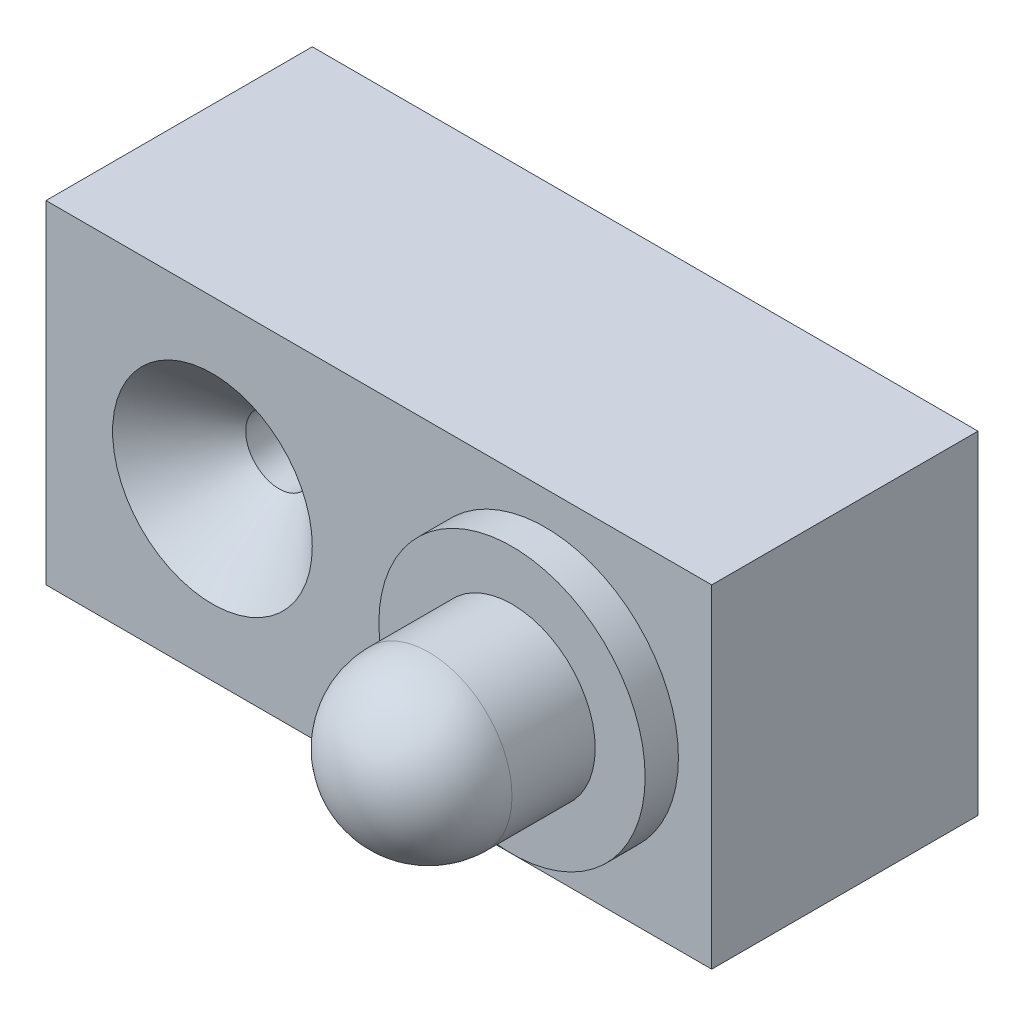
SolidWorks part; units mm, degrees
ref_plane "前视基准面" through (0, 0, 0) normal (0, 0, 1) x (1, 0, 0)
ref_plane "上视基准面" through (0, 0, 0) normal (0, 1, 0) x (1, 0, 0)
ref_plane "右视基准面" through (0, 0, 0) normal (1, 0, 0) x (0, 0, -1)
sketch "草图1" plane through (0, 0, 0) normal (0, 0, 1) x (1, 0, 0)
  line L1 (0, 0) -> (20, 0)
  line L2 (0, 0) -> (0, 10)
  line L3 (0, 10) -> (20, 10)
  line L4 (20, 0) -> (20, 10)
extrude "凸台-拉伸1" add sketch "草图1" along normal blind 8
sketch "草图2" plane through (0, 0, 8) normal (0, 0, 1) x (1, 0, 0)
  line L0 (0, 0) -> (20, 0) construction
  line L1 (0, 10) -> (0, 0) construction
  circle A0 centre (5, 5) radius 1
  dimension "D1" = 2
  dimension "D2" = 5
  dimension "D3" = 5
extrude "切除-拉伸1" cut sketch "草图2" against normal blind 8
chamfer "倒角1" distance 2 angle 45 1 edges at (6, 5, 8)
sketch "草图3" plane through (0, 0, 8) normal (0, 0, 1) x (1, 0, 0)
  line L0 (20, 0) -> (20, 10) construction
  circle A0 centre (15, 5) radius 4
  dimension "D1" = 8
  dimension "D2" = 5
extrude "凸台-拉伸2" add sketch "草图3" along normal blind 1
sketch "草图4" plane through (0, 0, 9) normal (0, 0, 1) x (1, 0, 0)
  circle A0 centre (15, 5) radius 2.5
  dimension "D1" = 5
extrude "凸台-拉伸3" add sketch "草图4" along normal blind 5
fillet "圆角1" radius 2.5 1 edges at (17.5, 5, 14)
